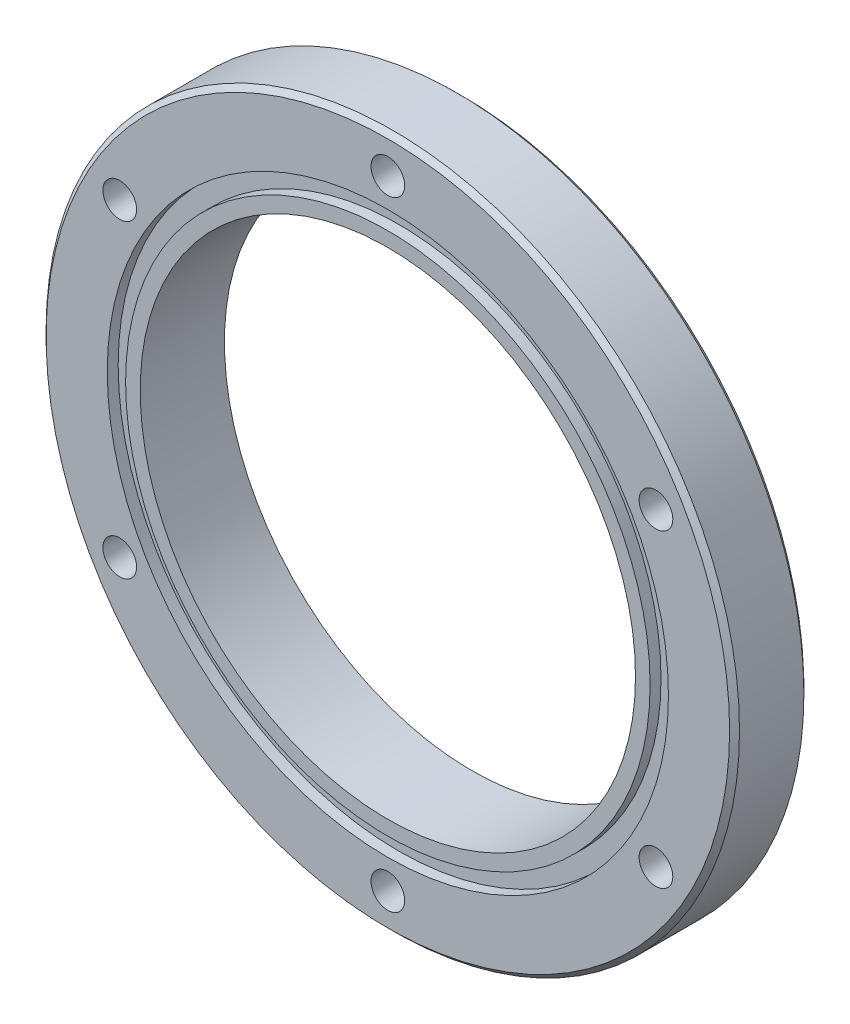
SolidWorks part; units mm, degrees
material "Q235B"
ref_plane "Front Plane" through (0, 0, 0) normal (0, 0, 1) x (1, 0, 0)
ref_plane "Top Plane" through (0, 0, 0) normal (0, 1, 0) x (1, 0, 0)
ref_plane "Right Plane" through (0, 0, 0) normal (1, 0, 0) x (0, 0, -1)
sketch "Sketch1" plane through (0, 0, 0) normal (0, 0, 1) x (1, 0, 0)
  circle A0 centre (0, 0) radius 70
  circle A1 centre (0, 0) radius 50
  circle A2 centre (0, 0) radius 62.5 construction
  dimension "D1" = 140
  dimension "D2" = 100
  dimension "D3" = 125
extrude "Boss-Extrude1" add sketch "Sketch1" along normal blind 17
sketch "Sketch2" plane through (0, 0, 17) normal (0, 0, 1) x (1, 0, 0)
  circle A0 centre (0, 0) radius 52.95
  circle A1 centre (0, 0) radius 56.65
  dimension "D1" = 105.9
  dimension "D2" = 113.3
extrude "Cut-Extrude1" cut sketch "Sketch2" against normal blind 2.2
sketch "Sketch3" plane through (0, 0, 0) normal (0, 0, -1) x (-1, 0, 0)
  circle A0 centre (0, 0) radius 51.5
  circle A1 centre (0, 0) radius 70 construction
  circle A2 centre (0, 0) radius 70
  dimension "D1" = 103
extrude "Cut-Extrude2" cut sketch "Sketch3" against normal blind 2
sketch "Sketch4" plane through (0, 0, 17) normal (0, 0, 1) x (1, 0, 0)
  circle A0 centre (0, 0) radius 62.5 construction
  circle A1 centre (0, 62.5) radius 3
  circle A2 centre (54.1266, 31.25) radius 3
  circle A3 centre (54.1266, -31.25) radius 3
  circle A4 centre (0, -62.5) radius 3
  circle A5 centre (-54.1266, -31.25) radius 3
  circle A6 centre (-54.1266, 31.25) radius 3
  dimension "D1" = 125
  dimension "D2" = 6
  dimension "D3" = 6
extrude "Cut-Extrude3" cut sketch "Sketch4" against normal blind 10
hole_wizard "M8 Tapped Hole1" positions "Sketch5" profile "Sketch6" tap size "M8" standard "GB"
sketch "Sketch5" plane through (0, 0, 17) normal (0, 0, 1) x (1, 0, 0)
  point P0 (0, 62.5)
  point P3 (54.1266, 31.25)
  point P6 (54.1266, -31.25)
  point P9 (0, -62.5)
  point P12 (-54.1266, -31.25)
  point P15 (-54.1266, 31.25)
cosmetic thread "Hole cosmetic thread1" parameters "D1"=10, "D2"=8
cosmetic thread "Hole cosmetic thread2" parameters "D1"=10, "D2"=8
cosmetic thread "Hole cosmetic thread3" parameters "D1"=10, "D2"=8
cosmetic thread "Hole cosmetic thread4" parameters "D1"=10, "D2"=8
cosmetic thread "Hole cosmetic thread5" parameters "D1"=10, "D2"=8
cosmetic thread "Hole cosmetic thread6" parameters "D1"=10, "D2"=8
sketch "Sketch6" plane through (0, 62.5, 17) normal (1, 0, 0) x (0, -1, 0)
  line L0 (0, 0) -> (0, 12.0429)
  line L1 (0, 12.0429) -> (3.4, 10)
  line L2 (3.4, 10) -> (3.4, 0)
  line L5 (3.4, 0) -> (0, 0)
  line L10 (0, 12.0429) -> (-3.4, 10) construction
  line L11 (0, -6.35) -> (0, 107.95) construction
  dimension "螺纹孔钻头直径" = 6.8
  dimension "螺纹孔钻头深度" = 10
  dimension "导头角度" = 118
chamfer "Chamfer1" distance 1 angle 45 2 edges at (-70, 0, 2) (70, 0, 17)
